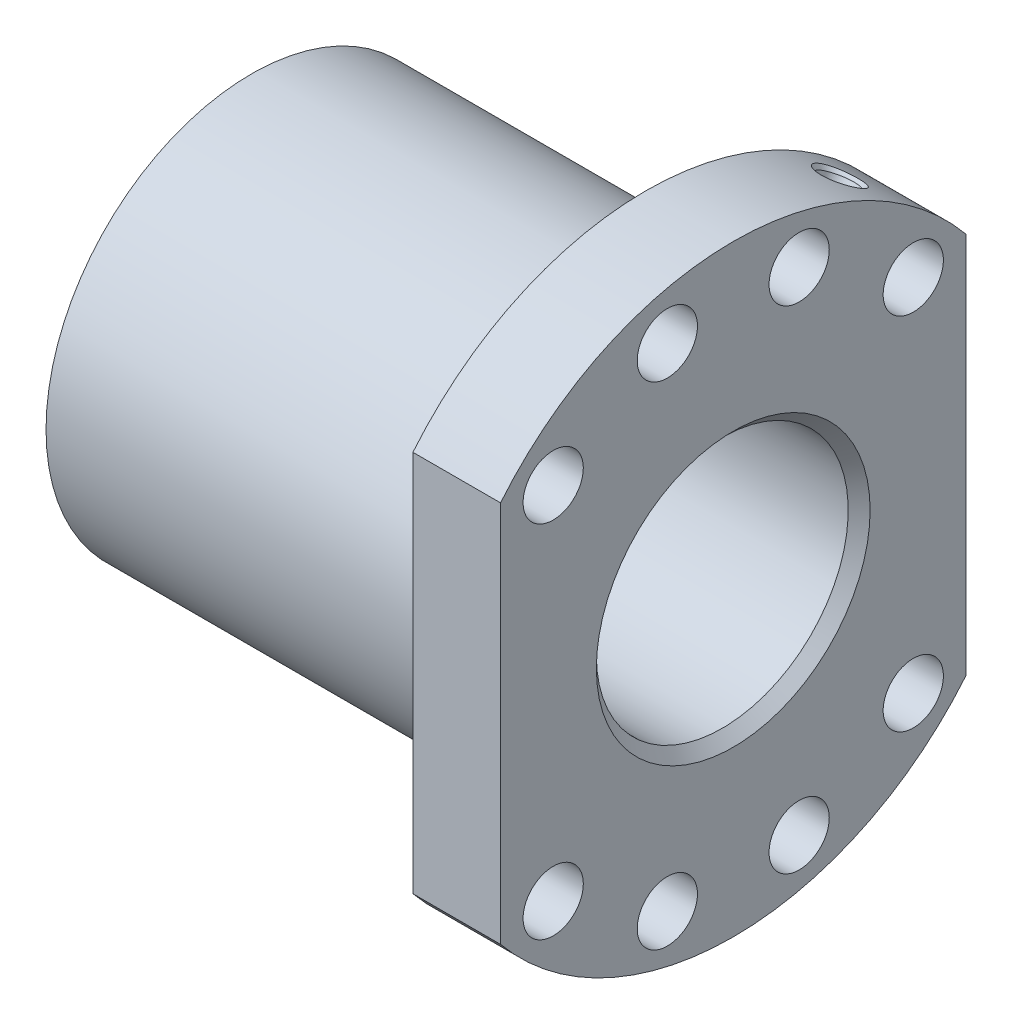
from build123d import *

# Parameters (mm, degrees)
CUT_EXTRUDE_1_DEPTH      = 88
CUT_EXTRUDE_1_DEPTH_BACK = 88
SKETCH_2_R               = 105
CUT_EXTRUDE_2_DEPTH      = 88
CUT_EXTRUDE_2_DEPTH_BACK = 88
SKETCH_3_R               = 5.5
CUT_EXTRUDE_3_DEPTH      = 88
CUT_EXTRUDE_3_DEPTH_BACK = 88
SKETCH_5_R               = 5.5
CUT_EXTRUDE_4_DEPTH      = 88
CUT_EXTRUDE_4_DEPTH_BACK = 88
SKETCH_6_R               = 5.5
CUT_EXTRUDE_5_DEPTH      = 88
CUT_EXTRUDE_5_DEPTH_BACK = 88
SKETCH_7_R               = 5.5
CUT_EXTRUDE_6_DEPTH      = 88
CUT_EXTRUDE_6_DEPTH_BACK = 88
SKETCH_8_R               = 5.5
CUT_EXTRUDE_7_DEPTH      = 88
CUT_EXTRUDE_7_DEPTH_BACK = 88
SKETCH_9_R               = 5.5
CUT_EXTRUDE_8_DEPTH      = 88
CUT_EXTRUDE_8_DEPTH_BACK = 88
SKETCH_10_R              = 5.5
CUT_EXTRUDE_9_DEPTH      = 88
CUT_EXTRUDE_9_DEPTH_BACK = 88
SKETCH_11_R              = 5.5


with BuildPart() as part:
    # 草图1 → 旋转1 (revolve)
    with BuildSketch(Plane.XY, mode=Mode.PRIVATE) as revolve_1_sk:
        Polygon((0, 37.5), (0, 25), (2, 23), (86, 23), (88, 25), (88, 55), (72, 55), (72, 37.5), align=None)
    revolve(revolve_1_sk.sketch.rotate(Axis((88, 0, 0), (-1, 0, 0)), 270), axis=Axis((88, 0, 0), (-1, 0, 0)))

    # 草图2 → 切除-拉伸1 (cut, two sides: drawn at the far end of the back side and taken through both)
    with BuildSketch(Plane(origin=(0, 0, 0), x_dir=(0, 0, -1), z_dir=(1, 0, 0)).offset(-CUT_EXTRUDE_1_DEPTH_BACK)):
        Circle(SKETCH_2_R)
        with BuildLine():
            Line((-42.5, 82.720916339), (-42.5, -82.720916339))
            ThreePointArc((-42.5, -82.720916339), (0, -93), (42.5, -82.720916339))
            Line((42.5, -82.720916339), (42.5, 82.720916339))
            ThreePointArc((42.5, 82.720916339), (0, 93), (-42.5, 82.720916339))
        make_face(mode=Mode.SUBTRACT)
    extrude(amount=CUT_EXTRUDE_1_DEPTH + CUT_EXTRUDE_1_DEPTH_BACK, mode=Mode.SUBTRACT)

    # 草图3 → 切除-拉伸2 (cut, two sides: drawn at the far end of the back side and taken through both)
    with BuildSketch(Plane(origin=(0, 0, 0), x_dir=(0, 0, -1), z_dir=(1, 0, 0)).offset(-CUT_EXTRUDE_2_DEPTH_BACK)):
        with Locations((-32.880465325, 32.880465325)):
            Circle(SKETCH_3_R)
    extrude(amount=CUT_EXTRUDE_2_DEPTH + CUT_EXTRUDE_2_DEPTH_BACK, mode=Mode.SUBTRACT)

    # 草图5 → 切除-拉伸3 (cut, two sides: drawn at the far end of the back side and taken through both)
    with BuildSketch(Plane(origin=(0, 0, 0), x_dir=(0, 0, -1), z_dir=(1, 0, 0)).offset(-CUT_EXTRUDE_3_DEPTH_BACK)):
        with Locations((-12.035085597, 44.915550922)):
            Circle(SKETCH_5_R)
    extrude(amount=CUT_EXTRUDE_3_DEPTH + CUT_EXTRUDE_3_DEPTH_BACK, mode=Mode.SUBTRACT)

    # 草图6 → 切除-拉伸4 (cut, two sides: drawn at the far end of the back side and taken through both)
    with BuildSketch(Plane(origin=(0, 0, 0), x_dir=(0, 0, -1), z_dir=(1, 0, 0)).offset(-CUT_EXTRUDE_4_DEPTH_BACK)):
        with Locations((12.035085597, 44.915550922)):
            Circle(SKETCH_6_R)
    extrude(amount=CUT_EXTRUDE_4_DEPTH + CUT_EXTRUDE_4_DEPTH_BACK, mode=Mode.SUBTRACT)

    # 草图7 → 切除-拉伸5 (cut, two sides: drawn at the far end of the back side and taken through both)
    with BuildSketch(Plane(origin=(0, 0, 0), x_dir=(0, 0, -1), z_dir=(1, 0, 0)).offset(-CUT_EXTRUDE_5_DEPTH_BACK)):
        with Locations((32.880465325, 32.880465325)):
            Circle(SKETCH_7_R)
    extrude(amount=CUT_EXTRUDE_5_DEPTH + CUT_EXTRUDE_5_DEPTH_BACK, mode=Mode.SUBTRACT)

    # 草图8 → 切除-拉伸6 (cut, two sides: drawn at the far end of the back side and taken through both)
    with BuildSketch(Plane(origin=(0, 0, 0), x_dir=(0, 0, -1), z_dir=(1, 0, 0)).offset(-CUT_EXTRUDE_6_DEPTH_BACK)):
        with Locations((32.880465325, -32.880465325)):
            Circle(SKETCH_8_R)
    extrude(amount=CUT_EXTRUDE_6_DEPTH + CUT_EXTRUDE_6_DEPTH_BACK, mode=Mode.SUBTRACT)

    # 草图9 → 切除-拉伸7 (cut, two sides: drawn at the far end of the back side and taken through both)
    with BuildSketch(Plane(origin=(0, 0, 0), x_dir=(0, 0, -1), z_dir=(1, 0, 0)).offset(-CUT_EXTRUDE_7_DEPTH_BACK)):
        with Locations((12.035085597, -44.915550922)):
            Circle(SKETCH_9_R)
    extrude(amount=CUT_EXTRUDE_7_DEPTH + CUT_EXTRUDE_7_DEPTH_BACK, mode=Mode.SUBTRACT)

    # 草图10 → 切除-拉伸8 (cut, two sides: drawn at the far end of the back side and taken through both)
    with BuildSketch(Plane(origin=(0, 0, 0), x_dir=(0, 0, -1), z_dir=(1, 0, 0)).offset(-CUT_EXTRUDE_8_DEPTH_BACK)):
        with Locations((-12.035085597, -44.915550922)):
            Circle(SKETCH_10_R)
    extrude(amount=CUT_EXTRUDE_8_DEPTH + CUT_EXTRUDE_8_DEPTH_BACK, mode=Mode.SUBTRACT)

    # 草图11 → 切除-拉伸9 (cut, two sides: drawn at the far end of the back side and taken through both)
    with BuildSketch(Plane(origin=(0, 0, 0), x_dir=(0, 0, -1), z_dir=(1, 0, 0)).offset(-CUT_EXTRUDE_9_DEPTH_BACK)):
        with Locations((-32.880465325, -32.880465325)):
            Circle(SKETCH_11_R)
    extrude(amount=CUT_EXTRUDE_9_DEPTH + CUT_EXTRUDE_9_DEPTH_BACK, mode=Mode.SUBTRACT)

    # 草图12 → 切除-旋转1 (revolve, cut)
    with BuildSketch(Plane(origin=(80, 0, 0), x_dir=(0, 0, -1), z_dir=(1, 0, 0)), mode=Mode.PRIVATE) as cut_revolve_1_sk:
        Polygon((7.5, 12.990381057), (4.901923789, 14.490381057), (16.901923789, 35.274990748), (16.621764571, 35.436740748), (24.283514571, 48.707281022), (24.035898385, 49.631397208), (27.5, 47.631397208), align=None)
    revolve(cut_revolve_1_sk.sketch.rotate(Axis((80, 47.631397208, -27.5), (0, -0.8660254037844387, 0.49999999999999983)), 180), axis=Axis((80, 47.631397208, -27.5), (0, -0.8660254037844387, 0.49999999999999983)), mode=Mode.SUBTRACT)


solid = part.part
